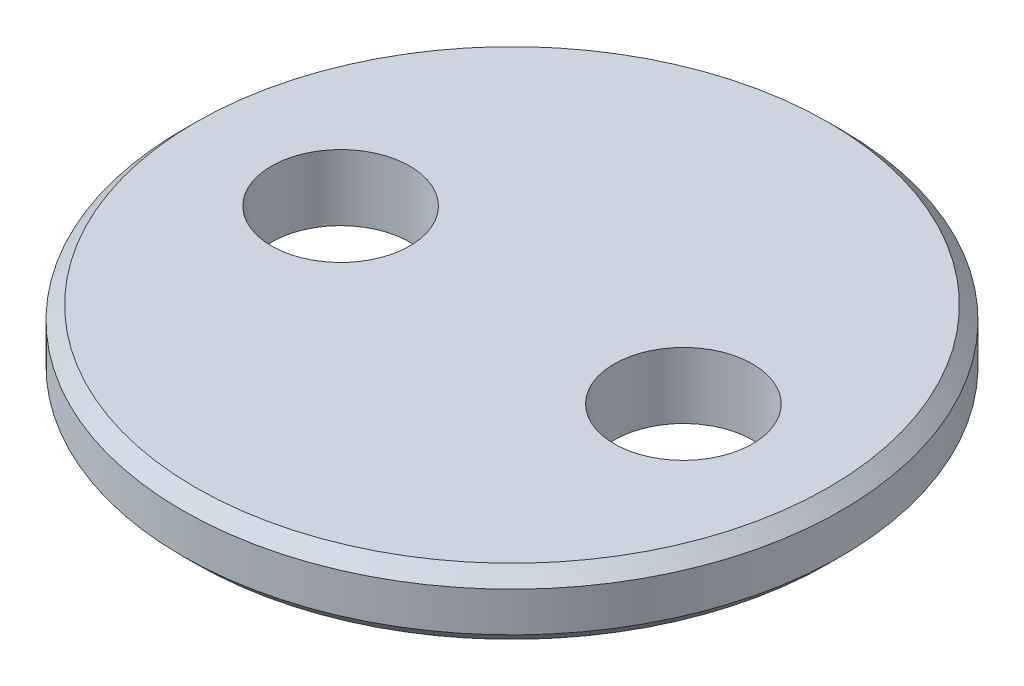
SolidWorks part; units mm, degrees
ref_plane "Front Plane" through (0, 0, 0) normal (0, 0, 1) x (1, 0, 0)
ref_plane "Top Plane" through (0, 0, 0) normal (0, 1, 0) x (1, 0, 0)
ref_plane "Right Plane" through (0, 0, 0) normal (1, 0, 0) x (0, 0, -1)
sketch "Sketch1" plane through (0, 0, 0) normal (0, 1, 0) x (1, 0, 0)
  line L0 (0, 0) -> (0, 15.7906) construction
  circle A0 centre (0, 0) radius 25
  circle A1 centre (-13, 0) radius 5.25
  circle A2 centre (13, 0) radius 5.25
  dimension "D1" = 50
  dimension "D2" = 26
  dimension "D3" = 10.5
extrude "Boss-Extrude1" add sketch "Sketch1" along normal blind 5
chamfer "Chamfer1" distance 1 angle 45 2 edges at (0, 0, 25) (0, 5, 25)
